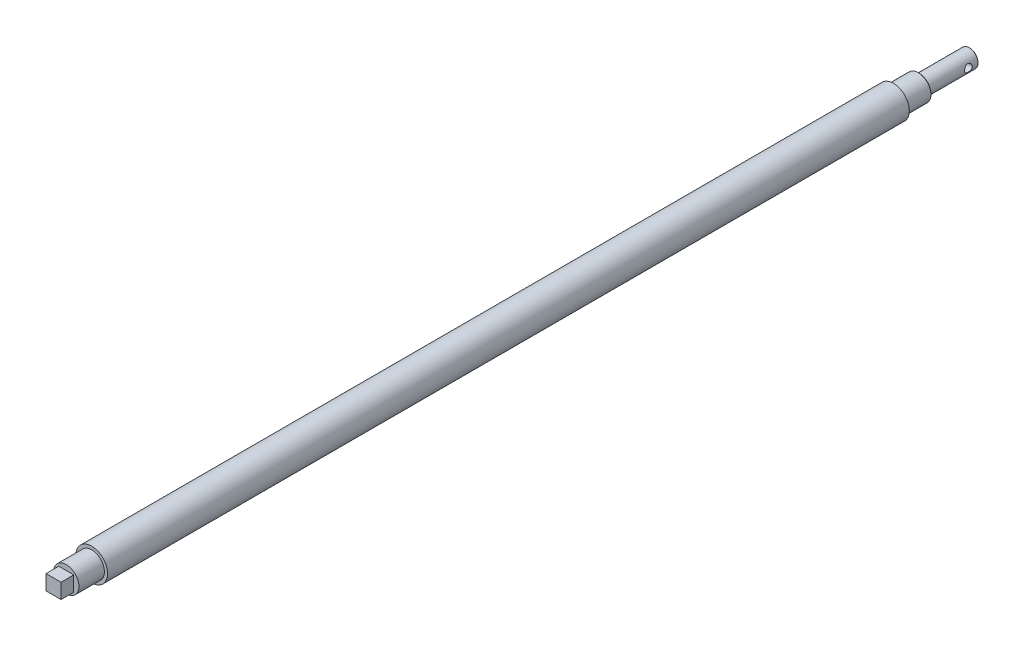
from build123d import *

# Parameters (mm, degrees)
SKETCH_1_R               = 12.5
EXTRUDE_1_DEPTH          = 315
SKETCH_2_R               = 10
EXTRUDE_2_DEPTH          = 30
EXTRUDE_START            = 20
SKETCH_3_R               = 10
EXTRUDE_3_DEPTH          = 20
CHAMFER_1_SIZE           = 0.5
SKETCH_4_R               = 7
EXTRUDE_4_DEPTH          = 40
CHAMFER_2_SIZE           = 0.5
CUT_EXTRUDE_1_DEPTH      = 376.416435442
CUT_EXTRUDE_1_DEPTH_BACK = 376.416435442
SKETCH_5_R               = 3
SKETCH_6_R               = 16.937839691
SKETCH_6_W               = 11.8
SKETCH_6_H               = 11.8
CUT_EXTRUDE_2_DEPTH      = 10


with BuildPart() as part:
    # 草图1 → 凸台-拉伸1 (new, symmetric)
    with BuildSketch(Plane.XY):
        Circle(SKETCH_1_R)
    extrude(amount=EXTRUDE_1_DEPTH, both=True)

    # 草图2 → 凸台-拉伸2 (add)
    with BuildSketch(Plane.XY.offset(315)):
        Circle(SKETCH_2_R)
    extrude(amount=EXTRUDE_2_DEPTH)

    # 草图3 → 凸台-拉伸3 (add)
    with BuildSketch(Plane(origin=(0, 0, -315), x_dir=(-1, 0, 0), z_dir=(0, 0, -1)).offset(EXTRUDE_START)):
        with Locations(Location((0, 0, 0), (0, 0, 180))):
            Circle(SKETCH_3_R)
    extrude(amount=-EXTRUDE_3_DEPTH)

    # 倒角1
    chamfer_1_edges = [part.edges().sort_by_distance(p)[0] for p in [
        (-10, 0, -335),
        (-10, 0, 345),
    ]]
    chamfer(chamfer_1_edges, length=CHAMFER_1_SIZE)

    # 草图4 → 凸台-拉伸4 (add)
    with BuildSketch(Plane(origin=(0, 0, -335), x_dir=(-1, 0, 0), z_dir=(0, 0, -1))):
        Circle(SKETCH_4_R)
    extrude(amount=EXTRUDE_4_DEPTH)

    # 倒角2
    chamfer_2_edges = [part.edges().sort_by_distance(p)[0] for p in [
        (7, 0, -375),
    ]]
    chamfer(chamfer_2_edges, length=CHAMFER_2_SIZE)

    # 草图5 → 切除-拉伸1 (cut, two sides: drawn at the far end of the back side and taken through both)
    with BuildSketch(Plane(origin=(0, 0, 0), x_dir=(0, 0, -1), z_dir=(1, 0, 0)).offset(-CUT_EXTRUDE_1_DEPTH_BACK)):
        with Locations((367, 0)):
            Circle(SKETCH_5_R)
    extrude(amount=CUT_EXTRUDE_1_DEPTH + CUT_EXTRUDE_1_DEPTH_BACK, mode=Mode.SUBTRACT)

    # 草图6 → 切除-拉伸2 (cut)
    with BuildSketch(Plane.XY.offset(345)):
        Circle(SKETCH_6_R)
        Rectangle(SKETCH_6_W, SKETCH_6_H, mode=Mode.SUBTRACT)
    extrude(amount=-CUT_EXTRUDE_2_DEPTH, mode=Mode.SUBTRACT)


solid = part.part
